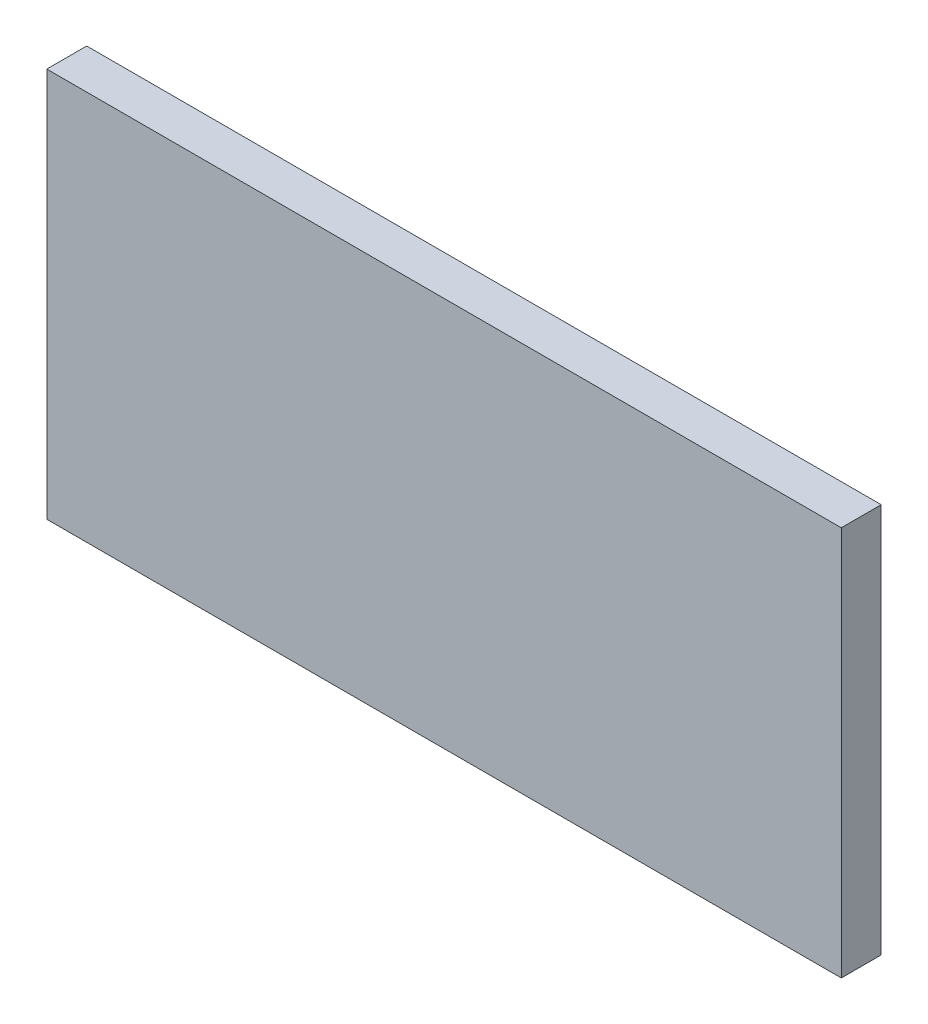
SolidWorks part; units mm, degrees
ref_plane "前视基准面" through (0, 0, 0) normal (0, 0, 1) x (1, 0, 0)
ref_plane "上视基准面" through (0, 0, 0) normal (0, 1, 0) x (1, 0, 0)
ref_plane "右视基准面" through (0, 0, 0) normal (1, 0, 0) x (0, 0, -1)
other "Configuration Table"
sketch "草图1" plane through (0, 0, 0) normal (0, 0, 1) x (1, 0, 0)
  line L1 (-24, 42) -> (374, 42)
  line L2 (-24, 42) -> (-24, -153.3186)
  line L3 (-24, -153.3186) -> (374, -153.3186)
  line L4 (374, 42) -> (374, -153.3186)
extrude "凸台-拉伸1" add sketch "草图1" along normal blind 20
